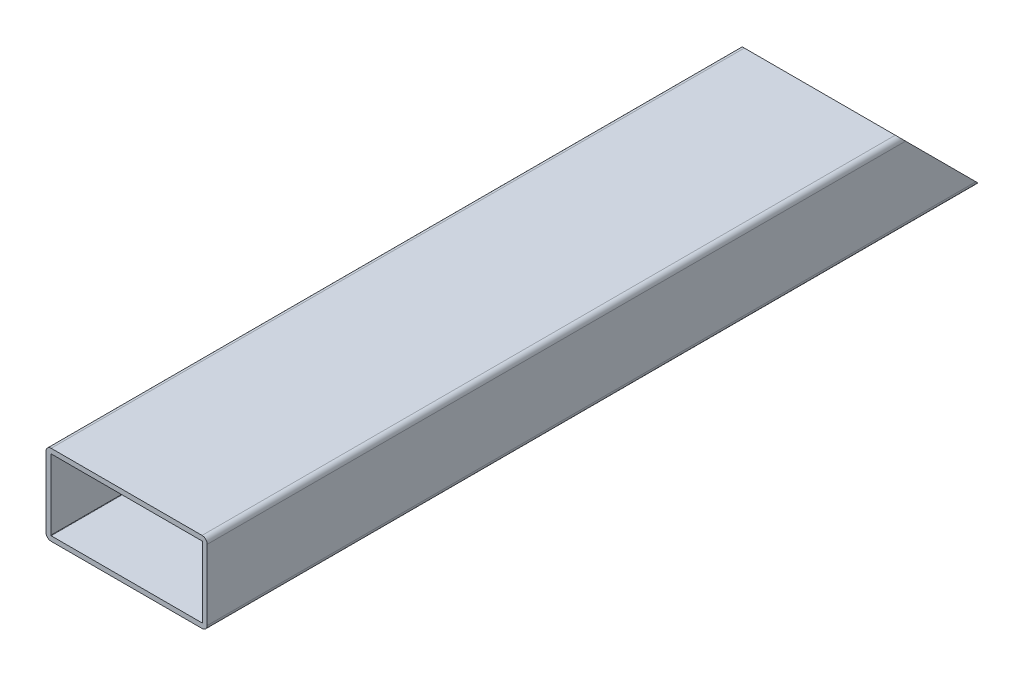
from build123d import *

# Parameters (mm, degrees)
EXTRUDE_1_DEPTH     = 500
CUT_EXTRUDE_1_DEPTH = 480


with BuildPart() as part:
    # 草图1 → 凸台-拉伸1 (new body)
    with BuildSketch(Plane.XY):
        with BuildLine():
            Line((-46.8, 25), (46.8, 25))
            ThreePointArc((46.8, 25), (49.0627417, 24.0627417), (50, 21.8))
            Line((50, 21.8), (50, -21.8))
            ThreePointArc((50, -21.8), (49.0627417, -24.0627417), (46.8, -25))
            Line((46.8, -25), (-46.8, -25))
            ThreePointArc((-46.8, -25), (-49.0627417, -24.0627417), (-50, -21.8))
            Line((-50, -21.8), (-50, 21.8))
            ThreePointArc((-50, 21.8), (-49.0627417, 24.0627417), (-46.8, 25))
        make_face()
        with BuildLine():
            Line((-46.8, 22), (46.8, 22))
            ThreePointArc((46.8, 22), (46.941421356, 21.941421356), (47, 21.8))
            Line((47, 21.8), (47, -21.8))
            ThreePointArc((47, -21.8), (46.941421356, -21.941421356), (46.8, -22))
            Line((46.8, -22), (-46.8, -22))
            ThreePointArc((-46.8, -22), (-46.941421356, -21.941421356), (-47, -21.8))
            Line((-47, -21.8), (-47, 21.8))
            ThreePointArc((-47, 21.8), (-46.941421356, 21.941421356), (-46.8, 22))
        make_face(mode=Mode.SUBTRACT)
    extrude(amount=EXTRUDE_1_DEPTH)

    # 草图3 → 切除-拉伸1 (cut)
    with BuildSketch(Plane(origin=(50, 0, 0), x_dir=(0, 0, -1), z_dir=(1, 0, 0))):
        Polygon((-70, 25), (-20, -25), (18.010342751, -26.423264748), (18.010342751, 25), align=None)
    extrude(amount=-CUT_EXTRUDE_1_DEPTH, mode=Mode.SUBTRACT)


solid = part.part
